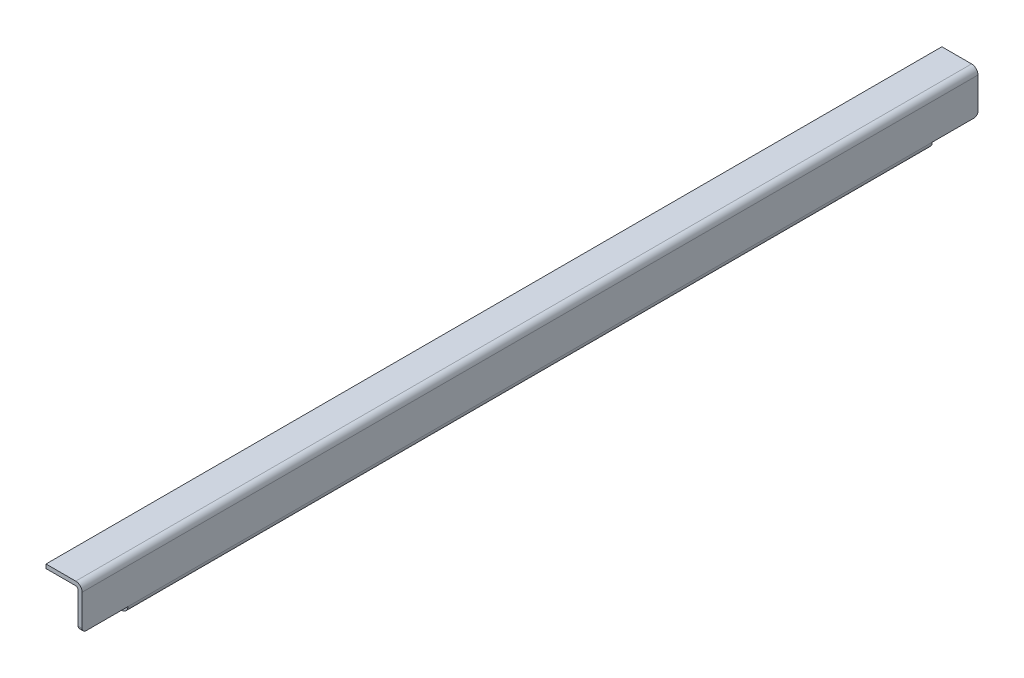
SolidWorks part; units mm, degrees
material "1023 碳钢板 (SS)"
ref_plane "Front Plane" through (0, 0, 0) normal (0, 0, 1) x (1, 0, 0)
ref_plane "Top Plane" through (0, 0, 0) normal (0, 1, 0) x (1, 0, 0)
ref_plane "Right Plane" through (0, 0, 0) normal (1, 0, 0) x (0, 0, -1)
sketch "Sketch1" plane through (0, 0, 0) normal (0, 0, 1) x (1, 0, 0)
  line L0 (0, 0) -> (37, 0)
  line L1 (45, -8) -> (45, -52)
  line L2 (37, -60) -> (0, -60)
  line L3 (0, -5) -> (37, -5)
  line L4 (40, -8) -> (40, -52)
  line L5 (37, -55) -> (0, -55)
  line L6 (0, 0) -> (0, -5)
  line L7 (0, -55) -> (0, -60)
  arc A0 (45, -52) -> (37, -60) centre (37, -52) cw
  arc A1 (37, 0) -> (45, -8) centre (37, -8) cw
  arc A2 (37, -5) -> (40, -8) centre (37, -8) cw
  arc A3 (40, -52) -> (37, -55) centre (37, -52) cw
  point P7 (45, -60)
  point P10 (45, 0)
  dimension "D4" = 8
  dimension "D1" = 45
  dimension "D2" = 60
  dimension "D3" = 45
  dimension "D5" = 5
extrude "Boss-Extrude1" add sketch "Sketch1" along normal blind 1116 contours L7 L2 A0 L1 A1 L0 L6 L3 A2 L4 A3 L5
sketch "Sketch2" plane through (0, 0, 0) normal (-1, 0, 0) x (0, 0, 1)
  line L0 (1116, -60) -> (0, -60) construction
  line L1 (1059, -52) -> (1151.4751, -52)
  line L2 (1059, -52) -> (1059, -90.6467)
  line L3 (1059, -90.6467) -> (1151.4751, -90.6467)
  line L4 (1151.4751, -52) -> (1151.4751, -90.6467)
  line L5 (1059, -52) -> (1151.4751, -90.6467) construction
  line L6 (1059, -90.6467) -> (1151.4751, -52) construction
  line L7 (1116, -8) -> (1116, -52) construction
  line L8 (0, -8) -> (0, -52) construction
  line L9 (57, -96.8575) -> (-33.3973, -96.8575)
  line L10 (57, -96.8575) -> (57, -52)
  line L11 (57, -52) -> (-33.3973, -52)
  line L12 (-33.3973, -96.8575) -> (-33.3973, -52)
  line L13 (57, -96.8575) -> (-33.3973, -52) construction
  line L14 (57, -52) -> (-33.3973, -96.8575) construction
  point P0 (1105.2376, -71.3233)
  point P9 (11.8014, -74.4287)
  dimension "D1" = 8
  dimension "D2" = 57
  dimension "D3" = 57
  dimension "D4" = 8
extrude "Cut-Extrude1" cut sketch "Sketch2" against normal blind 1116
sketch "Sketch3" plane through (0, -55, 0) normal (0, 1, 0) x (1, 0, 0)
  line L0 (0, -1116) -> (37, -1116) construction
  line L3 (0, -1059) -> (0, -57) construction
  circle A1 centre (12.5, -1024) radius 4
  dimension "D2" = 8
  dimension "D4" = 92
  dimension "D5" = 12.5
extrude "Cut-Extrude2" cut sketch "Sketch3" against normal blind 1116
fillet "Fillet1" radius 5 2 edges at (42.5, -52, 0) (42.5, -52, 1116)
hole_wizard "M10 Tapped Hole1" positions "Sketch4" profile "Sketch5" tap size "M10" standard "ISO"
sketch "Sketch4" plane through (0, -55, 0) normal (0, 1, 0) x (1, 0, 0)
  point P0 (12.5, -1024)
sketch "Sketch5" plane through (12.5, -55, 1024) normal (1, 0, 0) x (0, 0, 1)
  line L0 (0, 0) -> (0, 27.0537)
  line L1 (0, 27.0537) -> (4.25, 24.5)
  line L2 (4.25, 24.5) -> (4.25, 0)
  line L5 (4.25, 0) -> (0, 0)
  line L10 (0, 27.0537) -> (-4.25, 24.5) construction
  line L11 (0, -6.35) -> (0, 107.95) construction
  dimension "螺纹孔钻头直径" = 8.5
  dimension "螺纹孔钻头深度" = 24.5
  dimension "导头角度" = 118
cosmetic thread "Hole Thread Line1" parameters "D1"=20, "D2"=10
